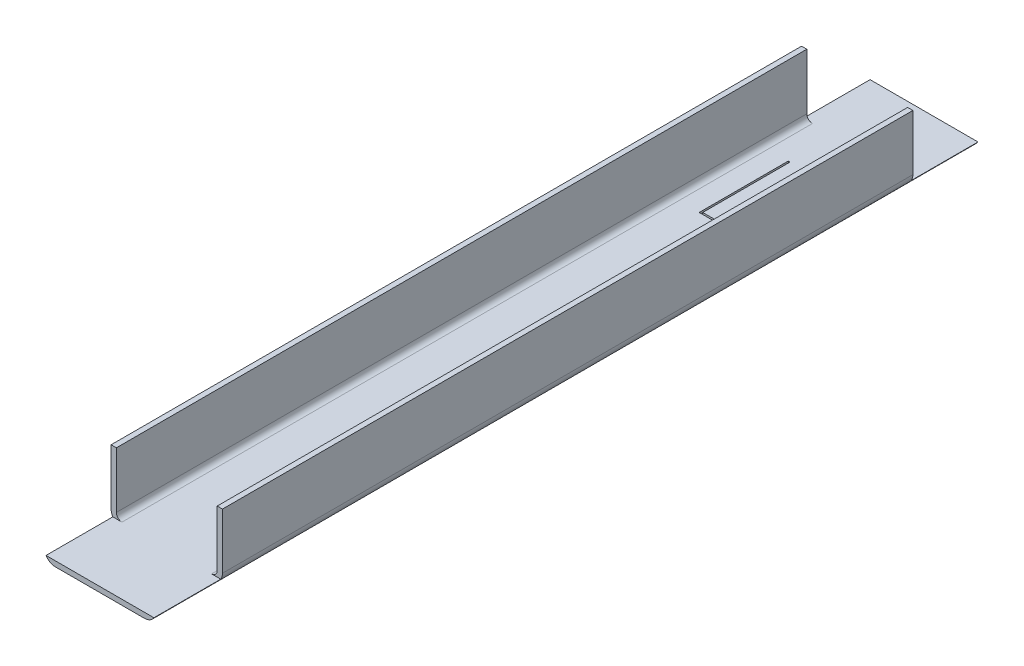
from build123d import *

# Parameters (mm, degrees)
BOSS_EXTRUDE1_DEPTH = 234.95
SKETCH2_W           = 19.05
SKETCH2_H           = 17.55
CUT_EXTRUDE1_DEPTH  = 238.849674164
CUT_EXTRUDE2_DEPTH  = 238.849674164


with BuildPart() as part:
    # Sketch1 → Boss-Extrude1 (new body)
    with BuildSketch(Plane.XY):
        with BuildLine():
            Line((30.25, 3.1), (30.25, 19.05))
            Line((30.25, 19.05), (31.75, 19.05))
            Line((31.75, 19.05), (31.75, 3.2))
            ThreePointArc((31.75, 3.2), (30.8127417, 0.9372583), (28.55, 0))
            Line((28.55, 0), (3.2, 0))
            ThreePointArc((3.2, 0), (0.9372583, 0.9372583), (0, 3.2))
            Line((0, 3.2), (0, 19.05))
            Line((0, 19.05), (1.5, 19.05))
            Line((1.5, 19.05), (1.5, 3.1))
            ThreePointArc((1.5, 3.1), (1.96862915, 1.96862915), (3.1, 1.5))
            Line((3.1, 1.5), (28.65, 1.5))
            ThreePointArc((28.65, 1.5), (29.78137085, 1.96862915), (30.25, 3.1))
        make_face()
    extrude(amount=BOSS_EXTRUDE1_DEPTH)

    # Sketch2 → Cut-Extrude1 (cut, through all)
    with BuildSketch(Plane(origin=(0, 0, 0), x_dir=(0, 0, -1), z_dir=(1, 0, 0))):
        with Locations((-9.525, 10.275)):
            Rectangle(SKETCH2_W, SKETCH2_H)
        with Locations((-225.425, 10.275)):
            Rectangle(SKETCH2_W, SKETCH2_H)
    extrude(amount=CUT_EXTRUDE1_DEPTH, mode=Mode.SUBTRACT)

    # Sketch3 → Cut-Extrude2 (cut, through all)
    with BuildSketch(Plane(origin=(0, 0, 0), x_dir=(1, 0, 0), z_dir=(0, 1, 0))):
        Polygon((22.821846385, -57.15), (8.928153615, -57.15), (8.928153615, -31.75), (9.428153615, -31.75), (9.428153615, -56.65), (22.321846385, -56.65), (22.321846385, -31.75), (22.821846385, -31.75), align=None)
    extrude(amount=CUT_EXTRUDE2_DEPTH, mode=Mode.SUBTRACT)


solid = part.part
